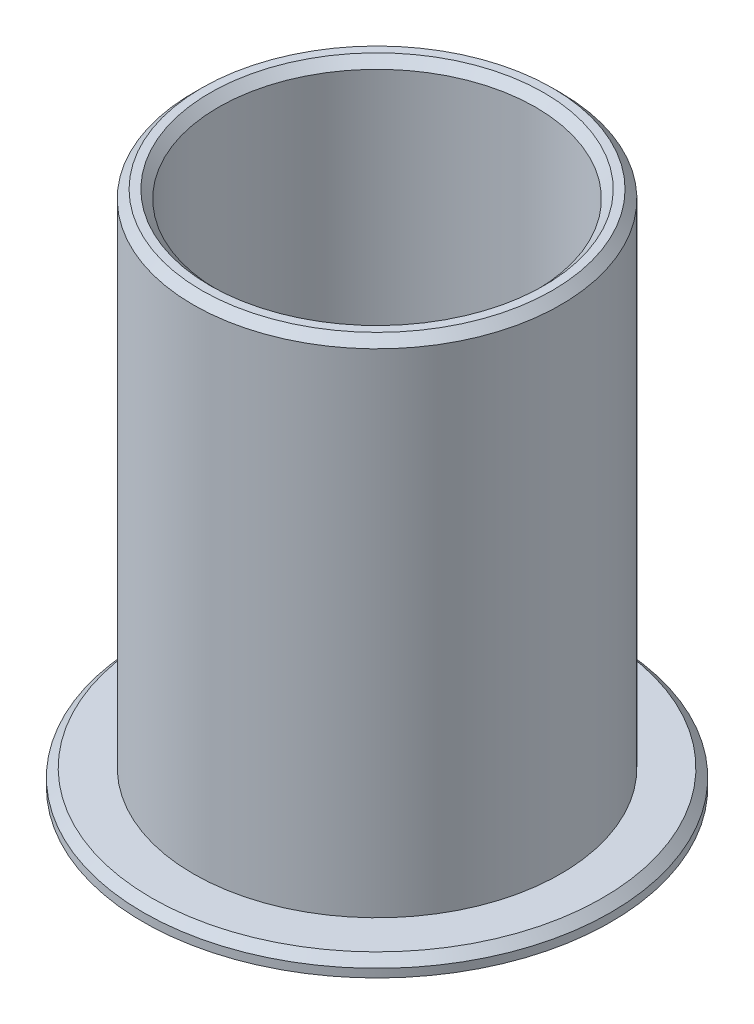
SolidWorks part; units mm, degrees
material "黑赛钢"
ref_plane "Front Plane" through (0, 0, 0) normal (0, 0, 1) x (1, 0, 0)
ref_plane "Top Plane" through (0, 0, 0) normal (0, 1, 0) x (1, 0, 0)
ref_plane "Right Plane" through (0, 0, 0) normal (1, 0, 0) x (0, 0, -1)
sketch "Sketch1" plane through (0, 0, 0) normal (0, 0, 1) x (1, 0, 0)
  line L0 (0, 0) -> (0, 71.9453) construction
  line L1 (9.5, 0) -> (14, 0)
  line L2 (14, 0) -> (14, 2)
  line L3 (14, 2) -> (11, 2)
  line L4 (11, 2) -> (11, 32)
  line L5 (11, 32) -> (9.5, 32)
  line L6 (9.5, 32) -> (9.5, 0)
  dimension "D1" = 9.5
  dimension "D2" = 11
  dimension "D3" = 32
  dimension "D4" = 2
  dimension "D5" = 14
revolve "Revolve1" add sketch "Sketch1" angle 360 about L0
chamfer "Chamfer1" distance 0.5 angle 45 4 edges at (0, 2, -14) (0, 32, -11) (0, 32, -9.5) (0, 0, -9.5)
chamfer "Chamfer2" distance 1 distance2 2 1 edges at (0, 0, -14)
